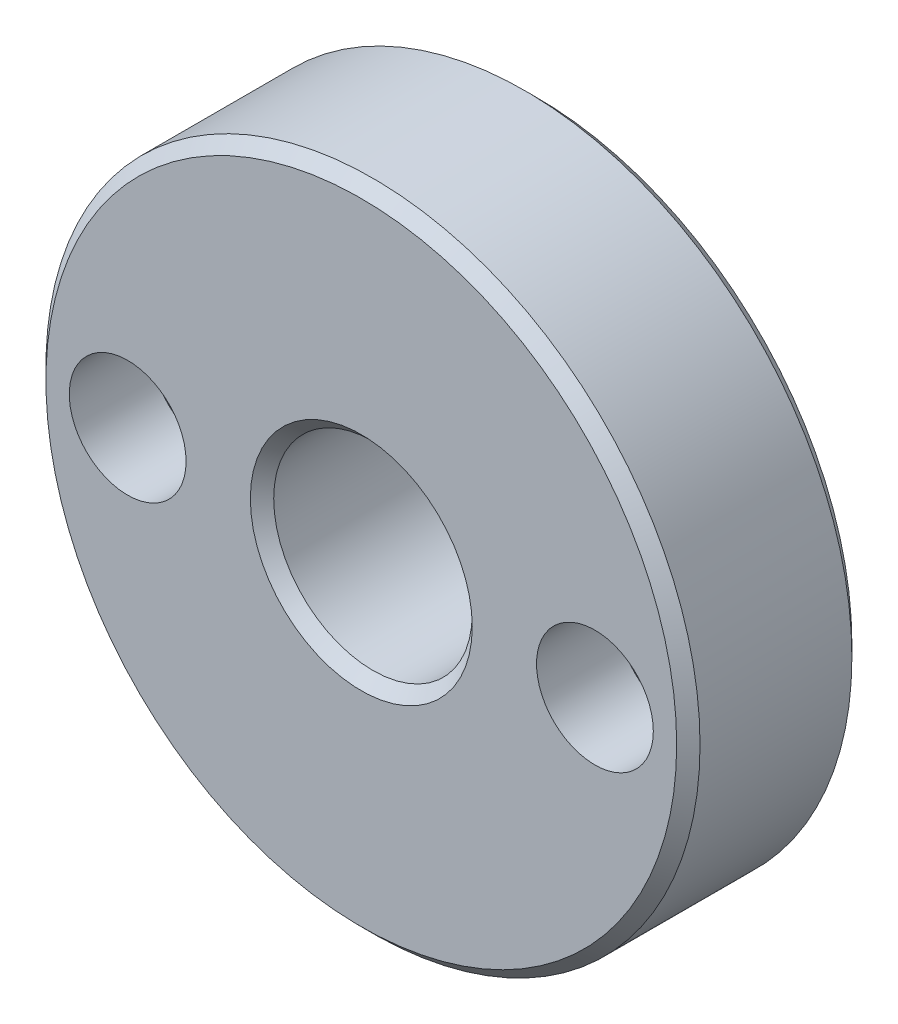
SolidWorks part; units mm, degrees
ref_plane "Front Plane" through (0, 0, 0) normal (0, 0, 1) x (1, 0, 0)
ref_plane "Top Plane" through (0, 0, 0) normal (0, 1, 0) x (1, 0, 0)
ref_plane "Right Plane" through (0, 0, 0) normal (1, 0, 0) x (0, 0, -1)
sketch "Sketch1" plane through (0, 0, 0) normal (0, 0, 1) x (1, 0, 0)
  circle A0 centre (0, 0) radius 28
extrude "Boss-Extrude1" add sketch "Sketch1" along normal blind 15
sketch "Sketch2" plane through (0, 0, 15) normal (0, 0, 1) x (1, 0, 0)
  line L0 (-20, 0) -> (20, 0)
  point P5 (0, 0)
hole_wizard "Hole1" positions "Sketch3" profile "Sketch4" legacy end condition through all
sketch "Sketch3" plane through (0, 0, 15) normal (0, 0, 1) x (1, 0, 0)
  point P0 (0, 0)
sketch "Sketch4" plane through (0, 0, 15) normal (1, 0, 0) x (0, -1, 0)
  line L0 (0, 0) -> (0, 15)
  line L1 (0, 15) -> (8.5, 15)
  line L2 (8.5, 15) -> (8.5, 0)
  line L3 (8.5, 0) -> (0, 0)
  line L4 (0, 110) -> (0, -10) construction
  dimension "直径" = 17
  dimension "深度" = 15
hole_wizard "Hole2" positions "Sketch5" profile "Sketch6" legacy end condition through all
sketch "Sketch5" plane through (0, 0, 15) normal (0, 0, 1) x (1, 0, 0)
  point P0 (-20, 0)
  point P3 (20, 0)
sketch "Sketch6" plane through (-20, 0, 15) normal (1, 0, 0) x (0, -1, 0)
  line L0 (0, 0) -> (0, 15)
  line L1 (0, 15) -> (2.75, 15)
  line L2 (2.75, 15) -> (2.75, 7)
  line L3 (2.75, 7) -> (5, 7)
  line L4 (5, 7) -> (5, 0)
  line L5 (5, 0) -> (0, 0)
  line L6 (0, 110) -> (0, -10) construction
  dimension "直径" = 5.5
  dimension "深度" = 15
  dimension "柱坑直径" = 10
  dimension "柱坑深度" = 7
chamfer "Chamfer1" distance 1 angle 45 4 edges at (28, 0, 0) (28, 0, 15) (8.5, 0, 15) (8.5, 0, 0)
